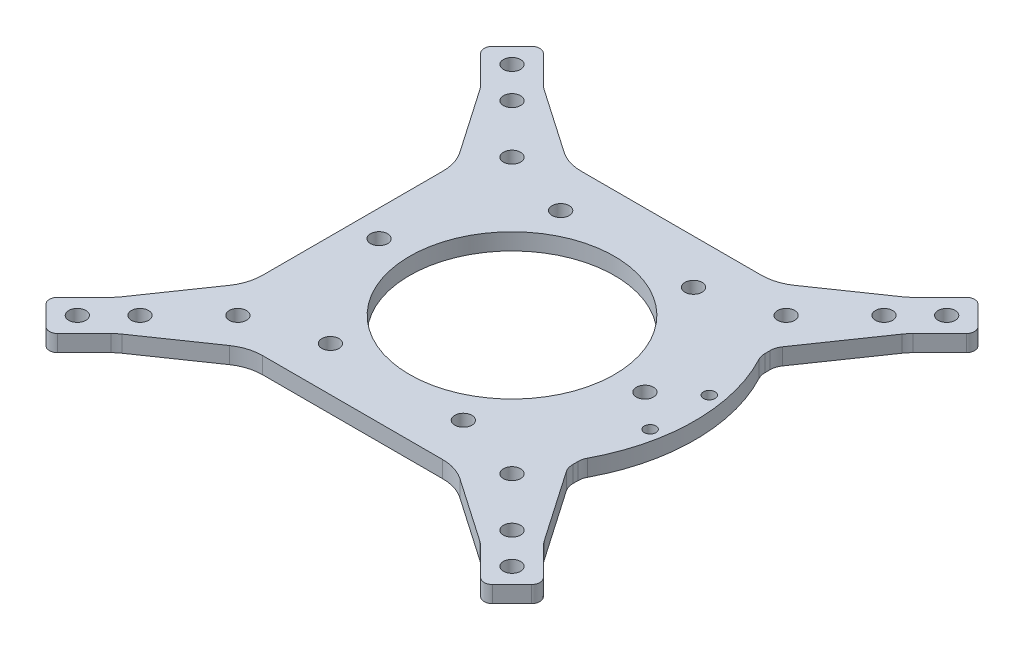
SolidWorks part; units mm, degrees
material "Thornel Mat VMA"
ref_plane "前视基准面" through (0, 0, 0) normal (0, 0, 1) x (1, 0, 0)
ref_plane "上视基准面" through (0, 0, 0) normal (0, 1, 0) x (1, 0, 0)
ref_plane "右视基准面" through (0, 0, 0) normal (1, 0, 0) x (0, 0, -1)
other "Configuration Table"
sketch "草图1" plane through (0, 0, 0) normal (0, 1, 0) x (1, 0, 0)
  line L0 (0, 0) -> (188.4122, 0) construction
  line L1 (0, 0) -> (0, 235.5594) construction
  line L2 (0, 152.028) -> (152.028, 0) construction
  line L3 (152.028, 0) -> (0, -152.028) construction
  line L4 (0, -152.028) -> (-152.028, 0) construction
  line L5 (-152.028, 0) -> (0, 152.028) construction
  line L6 (0, 0) -> (76.014, 76.014) construction
  line L8 (-10.6066, 141.4214) -> (-4.9497, 135.7645) construction
  line L9 (-141.4214, 10.6066) -> (-135.7645, 4.9497) construction
  line L10 (-4.9497, 135.7645) -> (-135.7645, 4.9497) construction
  line L11 (10.6066, 141.4214) -> (4.9497, 135.7645) construction
  line L12 (135.7645, 4.9497) -> (4.9497, 135.7645) construction
  line L13 (141.4214, 10.6066) -> (135.7645, 4.9497) construction
  line L14 (141.4214, -10.6066) -> (135.7645, -4.9497) construction
  line L15 (4.9497, -135.7645) -> (135.7645, -4.9497) construction
  line L16 (10.6066, -141.4214) -> (4.9497, -135.7645) construction
  line L17 (-10.6066, -141.4214) -> (-4.9497, -135.7645) construction
  line L18 (-135.7645, -4.9497) -> (-4.9497, -135.7645) construction
  line L19 (-141.4214, -10.6066) -> (-135.7645, -4.9497) construction
  line L20 (-24.7487, 24.7487) -> (24.7487, 24.7487) construction
  line L21 (-24.7487, 28.7987) -> (24.7487, 28.7987) construction
  line L22 (-24.7487, 20.6987) -> (24.7487, 20.6987) construction
  line L23 (-24.7487, 24.7487) -> (-24.7487, -24.7487) construction
  line L24 (-20.6987, 24.7487) -> (-20.6987, -24.7487) construction
  line L25 (-28.7987, 24.7487) -> (-28.7987, -24.7487) construction
  line L26 (24.7487, -24.7487) -> (-24.7487, -24.7487) construction
  line L27 (24.7487, -28.7987) -> (-24.7487, -28.7987) construction
  line L28 (24.7487, -20.6987) -> (-24.7487, -20.6987) construction
  line L29 (24.7487, 24.7487) -> (24.7487, -24.7487) construction
  line L30 (28.7987, 24.7487) -> (28.7987, -24.7487) construction
  line L31 (20.6987, 24.7487) -> (20.6987, -24.7487) construction
  line L36 (67.5287, 73.1856) -> (27.9307, 33.5876) construction
  line L37 (27.9307, 33.5876) -> (33.5876, 27.9307) construction
  line L38 (33.5876, 27.9307) -> (73.1856, 67.5287) construction
  line L39 (39.2444, 44.9013) -> (23.1419, 28.7987)
  line L40 (39.2444, 44.9013) -> (44.9013, 39.2444)
  line L41 (44.9013, 39.2444) -> (28.7987, 23.1419)
  line L42 (23.1419, 28.7987) -> (0, 28.7987)
  line L43 (28.7987, 23.1419) -> (28.7987, 0)
  line L44 (44.9013, -39.2444) -> (28.7987, -23.1419)
  line L45 (28.7987, -23.1419) -> (28.7987, 0)
  line L46 (44.9013, -39.2444) -> (39.2444, -44.9013)
  line L47 (39.2444, -44.9013) -> (23.1419, -28.7987)
  line L48 (23.1419, -28.7987) -> (0, -28.7987)
  line L49 (-39.2444, -44.9013) -> (-23.1419, -28.7987)
  line L50 (-23.1419, -28.7987) -> (0, -28.7987)
  line L51 (-39.2444, -44.9013) -> (-44.9013, -39.2444)
  line L52 (-44.9013, -39.2444) -> (-28.7987, -23.1419)
  line L53 (-28.7987, -23.1419) -> (-28.7987, 0)
  line L54 (-44.9013, 39.2444) -> (-28.7987, 23.1419)
  line L55 (-28.7987, 23.1419) -> (-28.7987, 0)
  line L56 (-44.9013, 39.2444) -> (-39.2444, 44.9013)
  line L57 (-39.2444, 44.9013) -> (-23.1419, 28.7987)
  line L58 (-23.1419, 28.7987) -> (0, 28.7987)
  line L59 (38.5373, 32.8805) -> (28.7987, 18.7487)
  line L60 (38.5373, 32.8805) -> (35.7089, 35.7089) construction
  line L61 (32.8805, 38.5373) -> (18.7487, 28.7987)
  line L62 (38.5373, -32.8805) -> (28.7987, -18.7487)
  line L63 (32.8805, -38.5373) -> (18.7487, -28.7987)
  line L64 (-32.8805, -38.5373) -> (-18.7487, -28.7987)
  line L65 (-38.5373, -32.8805) -> (-28.7987, -18.7487)
  line L66 (-38.5373, 32.8805) -> (-28.7987, 18.7487)
  line L67 (-32.8805, 38.5373) -> (-18.7487, 28.7987)
  circle A0 centre (0, 0) radius 18.5
  circle A1 centre (24, 0) radius 1.55
  circle A2 centre (12, -20.7846) radius 1.55
  circle A3 centre (-12, -20.7846) radius 1.55
  circle A4 centre (-24, 0) radius 1.55
  circle A5 centre (-12, 20.7846) radius 1.55
  circle A6 centre (12, 20.7846) radius 1.55
  circle A7 centre (0, -68) radius 32 construction
  circle A8 centre (24.7487, 24.7487) radius 1.55
  circle A9 centre (24.7487, -24.7487) radius 1.55
  circle A10 centre (-24.7487, -24.7487) radius 1.55
  circle A11 centre (-24.7487, 24.7487) radius 1.55
  arc A12 (-24.7487, 28.7987) -> (-24.7487, 20.6987) centre (-24.7487, 24.7487) ccw construction
  arc A13 (24.7487, 20.6987) -> (24.7487, 28.7987) centre (24.7487, 24.7487) ccw construction
  arc A14 (-20.6987, 24.7487) -> (-28.7987, 24.7487) centre (-24.7487, 24.7487) ccw construction
  arc A15 (-28.7987, -24.7487) -> (-20.6987, -24.7487) centre (-24.7487, -24.7487) ccw construction
  arc A16 (24.7487, -28.7987) -> (24.7487, -20.6987) centre (24.7487, -24.7487) ccw construction
  arc A17 (-24.7487, -20.6987) -> (-24.7487, -28.7987) centre (-24.7487, -24.7487) ccw construction
  arc A18 (28.7987, 24.7487) -> (20.6987, 24.7487) centre (24.7487, 24.7487) ccw construction
  arc A19 (20.6987, -24.7487) -> (28.7987, -24.7487) centre (24.7487, -24.7487) ccw construction
  circle A20 centre (39.2444, 39.2444) radius 1.55
  circle A21 centre (33.5876, 33.5876) radius 1.55
  circle A22 centre (24.7487, 24.7487) radius 3.75 construction
  circle A23 centre (39.2444, -39.2444) radius 1.55
  circle A24 centre (33.5876, -33.5876) radius 1.55
  circle A25 centre (-39.2444, -39.2444) radius 1.55
  circle A26 centre (-33.5876, -33.5876) radius 1.55
  circle A27 centre (-39.2444, 39.2444) radius 1.55
  circle A28 centre (-33.5876, 33.5876) radius 1.55
  point P24 (0, 0)
  point P27 (0, 24.7487)
  point P36 (0, 0)
  point P53 (0, 0)
  point P57 (-24.7487, 0)
  point P62 (0, -24.7487)
  point P68 (24.7487, 0)
  point P124 (0, 0)
  point P142 (0, 0)
  dimension "D2" = 37
  dimension "D3" = 24
  dimension "D4" = 3.1
  dimension "D7" = 64
  dimension "D8" = 35
  dimension "D9" = 3.1
  dimension "D15" = 2.5
  dimension "D18" = 8
  dimension "D21" = 7.5
  dimension "D23" = 5
  dimension "D1" = 215
  dimension "D6" = 68
  dimension "D11" = 8
  dimension "D12" = 15
  dimension "D13" = 15
  dimension "D16" = 8
  dimension "D17" = 56
  dimension "D19" = 4
  dimension "D20" = 4
  dimension "D24" = 6
  dimension "D5" = 6
  dimension "D10" = 4
  dimension "D14" = 4
  dimension "D22" = 4
  dimension "D25" = 4
extrude "凸台-拉伸1" add sketch "草图1" along normal blind 3 contours L58 L57 L56 L54 L55 L53 L52 L51 L49 L50 L48 L47 L46 L44 L45 L43 L41 L40 L39 L42 A28 A27 A26 A25 A24 A23 A21 A20 A11 A10 A9 A8 A6 A5 A4 | L54 L66 L55 | L67 L57 L58 | L65 L52 L53 | L49 L64 L50 | L63 L47 L48 | L44 L62 L45 | L59 L41 L43 | L39 L61 L42
sketch "草图2" plane through (0, 3, 0) normal (0, 1, 0) x (1, 0, 0)
  line L0 (0, 0) -> (30.75, 0) construction
  line L1 (0, 0) -> (30.2828, 5.3397) construction
  line L2 (28.7987, 16.1131) -> (28.7987, -16.1131)
  line L4 (28.7987, -18.7487) -> (28.7987, 18.7487) construction
  circle A0 centre (30.2828, 5.3397) radius 1.05
  arc A2 (28.7987, -16.1131) -> (28.7987, 16.1131) centre (0, 0) ccw
  circle A3 centre (30.2828, -5.3397) radius 1.05
  dimension "D3" = 2.1
  dimension "D4" = 66
  dimension "D1" = 30.75
  dimension "D2" = 10
extrude "凸台-拉伸2" add sketch "草图2" against normal up to surface (3 mm away) up to face at (0, 0, 0)
fillet "圆角1" radius 1.5 8 edges at (39.2444, 1.5, -44.9013) (44.9013, 1.5, -39.2444) (44.9013, 1.5, 39.2444) (39.2444, 1.5, 44.9013) (-39.2444, 1.5, 44.9013) (-44.9013, 1.5, 39.2444) (-39.2444, 1.5, -44.9013) (-44.9013, 1.5, -39.2444)
fillet "圆角2" radius 8 14 edges at (38.5373, 1.5, 32.8805) (32.8805, 1.5, 38.5373) (18.7487, 1.5, 28.7987) (-18.7487, 1.5, 28.7987) (-32.8805, 1.5, 38.5373) (-38.5373, 1.5, 32.8805) (-28.7987, 1.5, 18.7487) (-28.7987, 1.5, -18.7487) (-38.5373, 1.5, -32.8805) (-32.8805, 1.5, -38.5373) (-18.7487, 1.5, -28.7987) (18.7487, 1.5, -28.7987) (32.8805, 1.5, -38.5373) (38.5373, 1.5, -32.8805)
fillet "圆角3" radius 3 4 edges at (28.7987, 1.5, 16.1131) (28.7987, 1.5, -16.1131) (28.7987, 1.5, -18.7487) (28.7987, 1.5, 18.7487)
